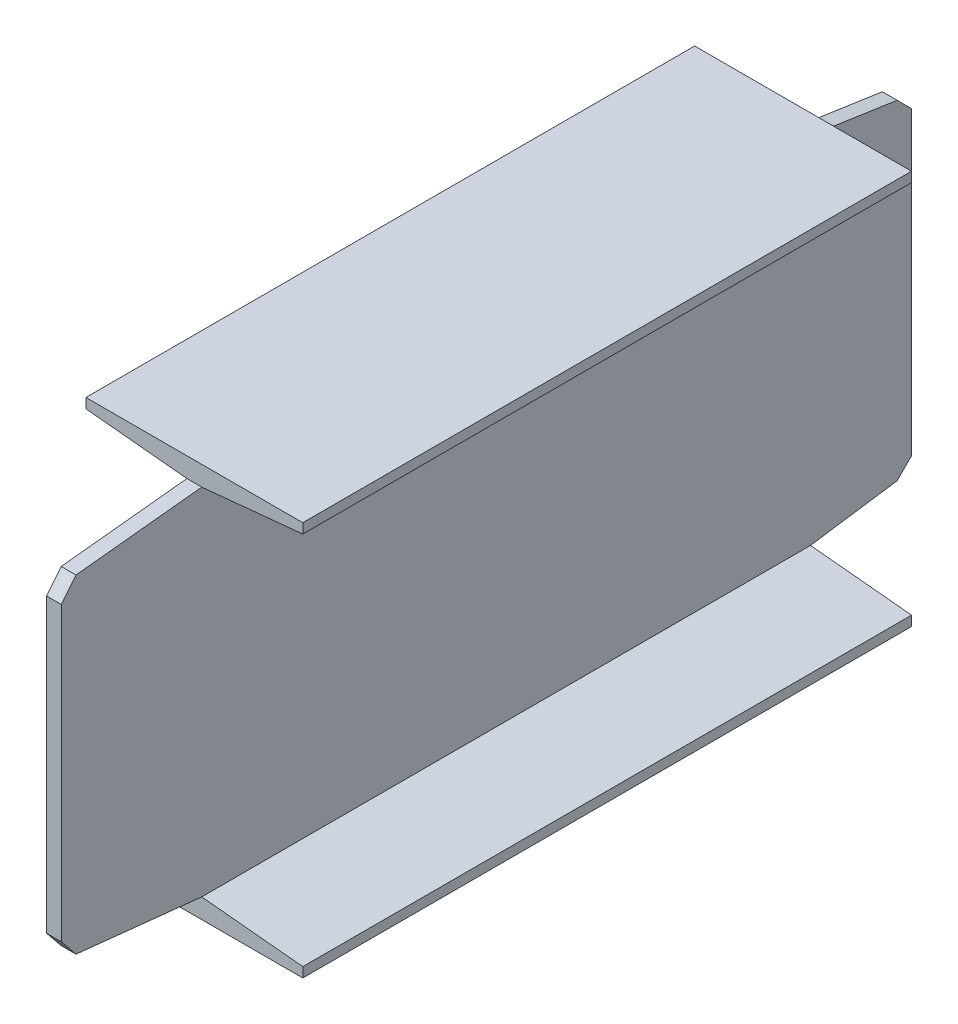
SolidWorks part; units mm, degrees
material "A3"
ref_plane "前视基准面" through (0, 0, 0) normal (0, 0, 1) x (1, 0, 0)
ref_plane "上视基准面" through (0, 0, 0) normal (0, 1, 0) x (1, 0, 0)
ref_plane "右视基准面" through (0, 0, 0) normal (1, 0, 0) x (0, 0, -1)
sketch "草图1" plane through (0, 0, 0) normal (0, 0, 1) x (1, 0, 0)
  line L0 (0, 80) -> (0, -80) construction
  line L1 (9.8926, 0) -> (-9.8926, 0) construction
  line L2 (44, 80) -> (-44, 80)
  line L3 (-44, 80) -> (-44, 76)
  line L4 (-44, 76) -> (-3, 72)
  line L5 (-3, 72) -> (-3, -72)
  line L6 (3, 72) -> (3, -72)
  line L7 (44, 76) -> (3, 72)
  line L8 (44, 80) -> (44, 76)
  line L9 (44, -80) -> (44, -76)
  line L10 (44, -76) -> (3, -72)
  line L11 (-44, -76) -> (-3, -72)
  line L12 (-44, -80) -> (-44, -76)
  line L13 (44, -80) -> (-44, -80)
  point P15 (0, 0)
  point P18 (3, 0)
  point P19 (-3, 0)
  dimension "D1" = 44
  dimension "D2" = 6
  dimension "D3" = 160
  dimension "D4" = 4
  dimension "D5" = 144
extrude "凸台-拉伸1" add sketch "草图1" along normal mid plane 345
sketch "草图3" plane through (0, 0, 0) normal (1, 0, 0) x (0, 0, -1)
  line L0 (-172.5, 66) -> (-115.5, 72)
  line L1 (-172.5, -72) -> (-172.5, 72) construction
  line L2 (-172.5, 72) -> (172.5, 72) construction
  line L3 (-115.5, 72) -> (-115.5, 80)
  line L4 (-172.5, 80) -> (172.5, 80) construction
  line L5 (-115.5, 80) -> (-172.5, 80)
  line L6 (-172.5, 80) -> (-172.5, 66)
  line L7 (0, 0) -> (0, 80) construction
  line L8 (172.5, 80) -> (172.5, 66)
  line L9 (131.5, 80) -> (172.5, 80)
  line L10 (131.5, 72) -> (131.5, 80)
  line L11 (172.5, 66) -> (131.5, 72)
  line L12 (0, 0) -> (172.5, 0) construction
  line L13 (172.5, -72) -> (172.5, 72) construction
  line L14 (172.5, -66) -> (131.5, -72)
  line L15 (131.5, -72) -> (131.5, -80)
  line L16 (131.5, -80) -> (172.5, -80)
  line L17 (172.5, -80) -> (172.5, -66)
  line L18 (-172.5, -80) -> (-172.5, -66)
  line L19 (-115.5, -80) -> (-172.5, -80)
  line L20 (-115.5, -72) -> (-115.5, -80)
  line L21 (-172.5, -66) -> (-115.5, -72)
  dimension "D1" = 57
  dimension "D2" = 66
  dimension "D3" = 41
extrude "切除-拉伸1" cut sketch "草图3" against normal through all both and the other way through all
chamfer "倒角1" distance 6 angle 45 2 edges at (0, -66, 172.5) (0, 66, 172.5)
chamfer "倒角2" distance 5 angle 45 2 edges at (0, -66, -172.5) (0, 66, -172.5)
